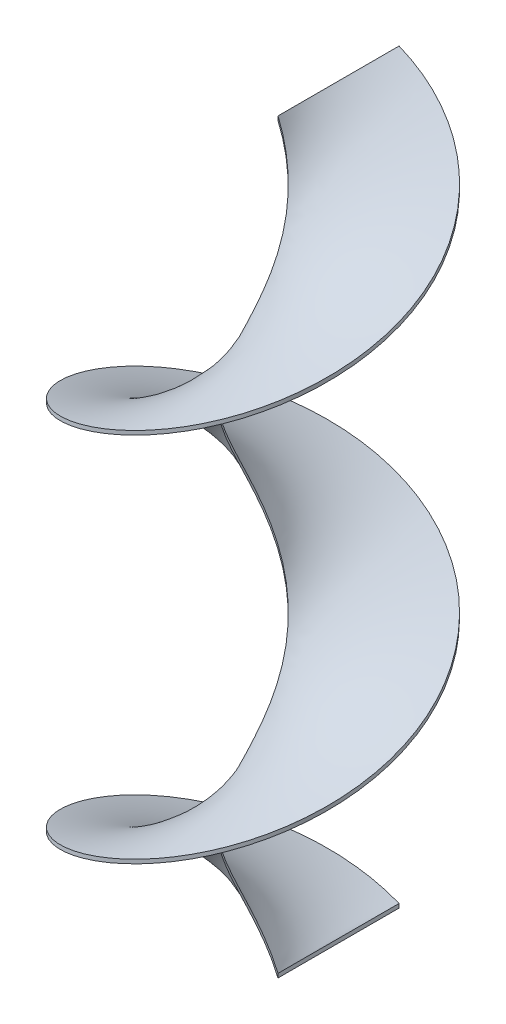
SolidWorks part; units mm, degrees
material "Q235A"
ref_plane "前视基准面" through (0, 0, 0) normal (0, 0, 1) x (1, 0, 0)
ref_plane "上视基准面" through (0, 0, 0) normal (0, 1, 0) x (1, 0, 0)
ref_plane "右视基准面" through (0, 0, 0) normal (1, 0, 0) x (0, 0, -1)
sketch "草图11" plane through (0, 0, 0) normal (1, 0, 0) x (0, 0, -1)
  line L0 (15.5, 0) -> (0, 0) construction
  line L1 (15.5, -1.25) -> (90.5, -1.25)
  line L2 (15.5, -1.25) -> (15.5, 1.25)
  line L3 (15.5, 1.25) -> (90.5, 1.25)
  line L4 (90.5, -1.25) -> (90.5, 1.25)
  dimension "D1" = 2.5
  dimension "D2" = 75
  dimension "D3" = 15.5
sketch "草图13" plane through (0, 0, 0) normal (0, 1, 0) x (1, 0, 0)
  circle A0 centre (0, 0) radius 15
  dimension "D1" = 30
curve "螺旋线/涡状线2" pitch 230 height 460 turns 2
sweep "扫描14" add profiles "草图11" path "螺旋线/涡状线2"
